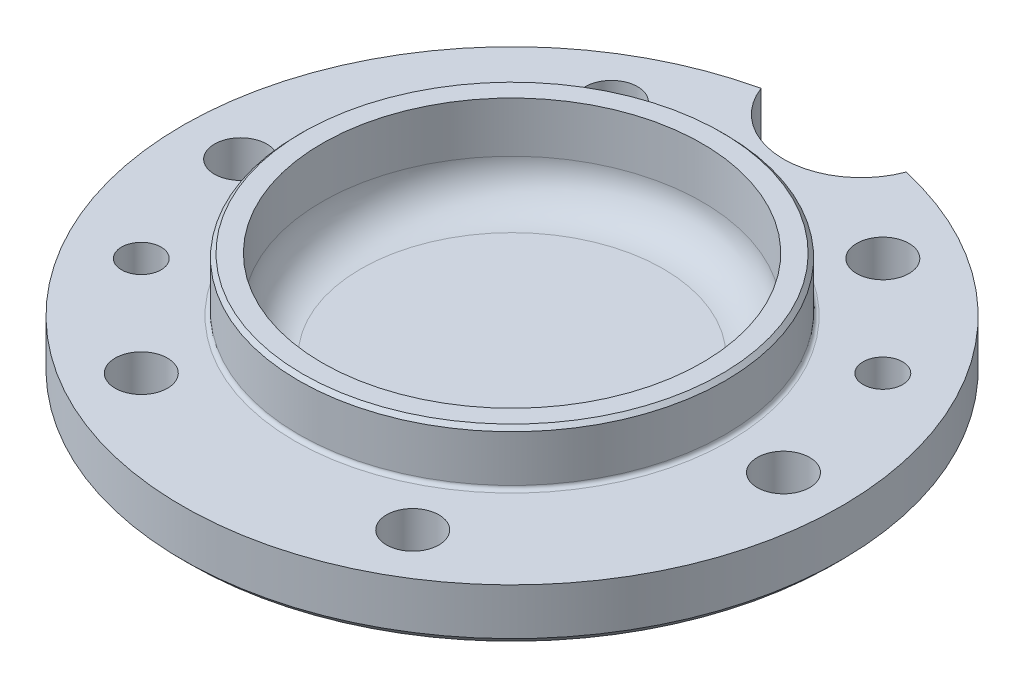
SolidWorks part; units mm, degrees
ref_plane "Front Plane" through (0, 0, 0) normal (0, 0, 1) x (1, 0, 0)
ref_plane "Top Plane" through (0, 0, 0) normal (0, 1, 0) x (1, 0, 0)
ref_plane "Right Plane" through (0, 0, 0) normal (1, 0, 0) x (0, 0, -1)
sketch "Sketch1" plane through (0, 0, 0) normal (0, 1, 0) x (1, 0, 0)
  circle A0 centre (0, 0) radius 85
  dimension "D1" = 170
extrude "Boss-Extrude1" add sketch "Sketch1" along normal blind 14
sketch "Sketch2" plane through (0, 14, 0) normal (0, 1, 0) x (1, 0, 0)
  circle A0 centre (0, 0) radius 55
  dimension "D1" = 110
extrude "Boss-Extrude2" add sketch "Sketch2" along normal blind 14
sketch "Sketch3" plane through (0, 28, 0) normal (0, 1, 0) x (1, 0, 0)
  circle A0 centre (0, 0) radius 49
  dimension "D1" = 98
extrude "Cut-Extrude1" cut sketch "Sketch3" against normal blind 23
fillet "Fillet1" radius 10 1 edges at (0, 5, 49)
fillet "Fillet2" radius 1 1 edges at (0, 14, 55)
chamfer "Chamfer1" distance 1 angle 45 1 edges at (0, 28, 55)
sketch "Sketch4" plane through (0, 14, 0) normal (0, 1, 0) x (1, 0, 0)
  line L0 (-35, 60.6218) -> (0, 0) construction
  line L1 (0, 0) -> (0, 132.1662) construction
  circle A0 centre (0, 0) radius 70 construction
  circle A1 centre (0, 90) radius 20
  circle A2 centre (-35, 60.6218) radius 6.75
  circle A3 centre (35, 60.6218) radius 6.75
  circle A4 centre (70, 0) radius 6.75
  circle A5 centre (35, -60.6218) radius 6.75
  circle A6 centre (-35, -60.6218) radius 6.75
  circle A7 centre (-70, 0) radius 6.75
  point P21 (0, 0)
  dimension "D1" = 140
  dimension "D2" = 40
  dimension "D4" = 13.5
  dimension "D3" = 90
  dimension "D5" = 30
  dimension "D6" = 6
extrude "Cut-Extrude2" cut sketch "Sketch4" against normal through all
sketch "Sketch5" plane through (0, 14, 0) normal (0, 1, 0) x (1, 0, 0)
  line L0 (0, 0) -> (-60.6218, -35) construction
  line L1 (-70, 0) -> (0, 0) construction
  line L2 (0, 0) -> (60.6218, 35) construction
  circle A0 centre (0, 0) radius 70 construction
  dimension "D1" = 30
hole_wizard "M12 Tapped Hole1" positions "Sketch6" profile "Sketch7" tap size "M12" standard "GB" end condition through all
sketch "Sketch6" plane through (0, 14, 0) normal (0, 1, 0) x (1, 0, 0)
  point P0 (-60.6218, -35)
  point P3 (60.6218, 35)
sketch "Sketch7" plane through (-60.6218, 14, 35) normal (1, 0, 0) x (0, 0, 1)
  line L0 (0, 0) -> (0, 14)
  line L1 (0, 14) -> (5.1, 14)
  line L2 (5.1, 14) -> (5.1, 0)
  line L5 (5.1, 0) -> (0, 0)
  line L11 (0, -6.35) -> (0, 107.95) construction
  dimension "通孔螺纹孔钻头直径" = 10.2
  dimension "通孔螺纹孔钻头深度" = 14
cosmetic thread "Cosmetic Thread1" parameters "D2"=12
cosmetic thread "Cosmetic Thread2" parameters "D2"=12
chamfer "Chamfer2" distance 2 angle 45 2 edges at (0, 0, -70) (0, 0, 85)
